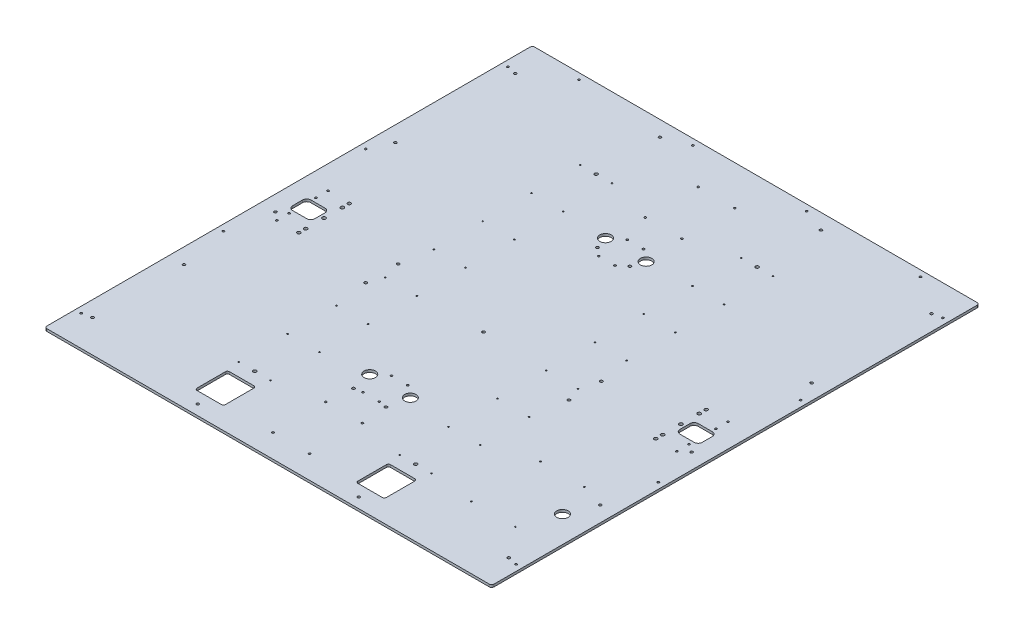
SolidWorks part; units mm, degrees
material "A3钢"
ref_plane "前视基准面" through (0, 0, 0) normal (0, 0, 1) x (1, 0, 0)
ref_plane "上视基准面" through (0, 0, 0) normal (0, 1, 0) x (1, 0, 0)
ref_plane "右视基准面" through (0, 0, 0) normal (1, 0, 0) x (0, 0, -1)
sketch "草图1" plane through (0, 0, 0) normal (0, 1, 0) x (1, 0, 0)
  line L1 (-550, 600) -> (550, 600)
  line L2 (-550, 600) -> (-550, -600)
  line L3 (-550, -600) -> (550, -600)
  line L4 (550, 600) -> (550, -600)
  line L5 (-550, 600) -> (550, -600) construction
  line L6 (-550, -600) -> (550, 600) construction
  point P0 (0, 0)
  dimension "D1" = 1100
  dimension "D2" = 1200
extrude "凸台-拉伸1" add sketch "草图1" along normal blind 6
fillet "圆角1" radius 6 4 edges at (-550, 3, -600) (550, 3, -600) (550, 3, 600) (-550, 3, 600)
hole_wizard "M6 螺纹孔1" positions "草图48" profile "草图50" tap size "M6" standard "GB" end condition through all
sketch "草图48" plane through (0, 0, 0) normal (0, -1, 0) x (-1, 0, 0)
  circle A0 centre (492, 39.5) radius 3.25 construction
  circle A1 centre (492, 9.5) radius 3.25 construction
  circle A2 centre (492, -56.5) radius 3.5 construction
  circle A3 centre (492, -86.5) radius 3.5 construction
  point P0 (492, -86.5)
  point P2 (492, -56.5)
  point P4 (492, 9.5)
  point P6 (492, 39.5)
sketch "草图50" plane through (-492, 0, 86.5) normal (1, 0, 0) x (0, 0, -1)
  line L0 (0, 0) -> (0, 6)
  line L1 (0, 6) -> (2.5, 6)
  line L2 (2.5, 6) -> (2.5, 0)
  line L5 (2.5, 0) -> (0, 0)
  line L11 (0, -6.35) -> (0, 107.95) construction
  dimension "通孔螺纹孔钻头直径" = 5
  dimension "通孔螺纹孔钻头深度" = 6
cosmetic thread "孔螺蚊线36" parameters "D2"=6
cosmetic thread "孔螺蚊线37" parameters "D2"=6
cosmetic thread "孔螺蚊线38" parameters "D2"=6
cosmetic thread "孔螺蚊线39" parameters "D2"=6
hole_wizard "Ø8.0 (8) 直径孔1" positions "草图51" profile "草图53" hole size "Ø8.0" standard "GB" end condition through all
sketch "草图51" plane through (0, 0, 0) normal (0, -1, 0) x (-1, 0, 0)
  point P0 (439, -85.5)
  point P3 (439, 38.5)
sketch "草图53" plane through (-439, 0, 85.5) normal (1, 0, 0) x (0, 0, -1)
  line L0 (0, 0) -> (0, 6)
  line L1 (0, 6) -> (4, 6)
  line L2 (4, 6) -> (4, 0)
  line L5 (4, 0) -> (0, 0)
  line L11 (0, -6.35) -> (0, 107.95) construction
  dimension "通孔孔直径" = 8
  dimension "通孔孔深度" = 6
hole_wizard "Ø8.5 (8.5) 直径孔1" positions "草图54" profile "草图55" hole size "Ø8.5" standard "GB" end condition through all
sketch "草图54" plane through (0, 0, 0) normal (0, -1, 0) x (-1, 0, 0)
  circle A0 centre (439, -68.5) radius 3.4 construction
  circle A1 centre (439, 21.5) radius 3.4 construction
  circle A2 centre (439, -23.5) radius 3.4 construction
  point P0 (439, 21.5)
  point P2 (439, -23.5)
  point P4 (439, -68.5)
sketch "草图55" plane through (-439, 0, -21.5) normal (1, 0, 0) x (0, 0, -1)
  line L0 (0, 0) -> (0, 6)
  line L1 (0, 6) -> (4.25, 6)
  line L2 (4.25, 6) -> (4.25, 0)
  line L5 (4.25, 0) -> (0, 0)
  line L11 (0, -6.35) -> (0, 107.95) construction
  dimension "通孔孔直径" = 8.5
  dimension "通孔孔深度" = 6
sketch "草图56" plane through (0, 6, 0) normal (0, 1, 0) x (1, 0, 0)
  line L0 (-439, -23.5) -> (-595.6745, -23.5) construction
  line L2 (-494, -1) -> (-459, -1)
  line L3 (-504, -11) -> (-504, -36)
  line L4 (-494, -46) -> (-459, -46)
  line L5 (-449, -11) -> (-449, -36)
  line L6 (-504, -1) -> (-449, -46) construction
  line L7 (-504, -46) -> (-449, -1) construction
  circle A0 centre (-439, -23.5) radius 4.25 construction
  arc A1 (-459, -1) -> (-449, -11) centre (-459, -11) cw
  arc A2 (-449, -36) -> (-459, -46) centre (-459, -36) cw
  arc A3 (-494, -46) -> (-504, -36) centre (-494, -36) cw
  arc A4 (-504, -11) -> (-494, -1) centre (-494, -11) cw
  point P3 (-476.5, -23.5)
  dimension "D4" = 10
  dimension "D1" = 10
  dimension "D2" = 55
  dimension "D3" = 45
extrude "切除-拉伸1" cut sketch "草图56" against normal blind 10
hole_wizard "Ø8.0 (8) 直径孔2" positions "草图63" profile "草图64" hole size "Ø8.0" standard "GB" end condition through all
sketch "草图63" plane through (0, 6, 0) normal (0, 1, 0) x (1, 0, 0)
  circle A0 centre (-198, 405) radius 4 construction
  circle A1 centre (-198, -435) radius 4 construction
  point P2 (-198, 405)
  point P7 (-198, -435)
sketch "草图64" plane through (-198, 6, -405) normal (1, 0, 0) x (0, 0, 1)
  line L0 (0, 0) -> (0, 6)
  line L1 (0, 6) -> (4, 6)
  line L2 (4, 6) -> (4, 0)
  line L5 (4, 0) -> (0, 0)
  line L11 (0, -6.35) -> (0, 107.95) construction
  dimension "通孔孔直径" = 8
  dimension "通孔孔深度" = 6
hole_wizard "M4 螺纹孔1" positions "草图65" profile "草图67" tap size "M4" standard "GB" end condition through all
sketch "草图65" plane through (0, 6, 0) normal (0, 1, 0) x (1, 0, 0)
  circle A0 centre (-237, -435) radius 2.25 construction
  circle A1 centre (-159, -435) radius 2.25 construction
  point P0 (-159, -435)
  point P2 (-237, -435)
sketch "草图67" plane through (-159, 6, 435) normal (1, 0, 0) x (0, 0, 1)
  line L0 (0, 0) -> (0, 6)
  line L1 (0, 6) -> (1.65, 6)
  line L2 (1.65, 6) -> (1.65, 0)
  line L5 (1.65, 0) -> (0, 0)
  line L11 (0, -6.35) -> (0, 107.95) construction
  dimension "通孔螺纹孔钻头直径" = 3.3
  dimension "通孔螺纹孔钻头深度" = 6
cosmetic thread "孔螺蚊线44" parameters "D2"=4
cosmetic thread "孔螺蚊线45" parameters "D2"=4
pattern_linear "阵列(线性)1" count 8 spacing 120 along (0, 0, -1) of "M4 螺纹孔1"
sketch "草图59" plane through (0, 6, 0) normal (0, 1, 0) x (1, 0, 0)
  line L0 (0, 0) -> (0, -646.723) construction
  line L1 (-544, -600) -> (544, -600) construction
  line L2 (-228, -467) -> (-168, -467)
  line L3 (-233, -472) -> (-233, -542)
  line L4 (-228, -547) -> (-168, -547)
  line L5 (-163, -472) -> (-163, -542)
  line L6 (-233, -467) -> (-163, -547) construction
  line L7 (-233, -547) -> (-163, -467) construction
  arc A0 (-168, -467) -> (-163, -472) centre (-168, -472) cw
  arc A1 (-163, -542) -> (-168, -547) centre (-168, -542) cw
  arc A2 (-228, -547) -> (-233, -542) centre (-228, -542) cw
  arc A3 (-233, -472) -> (-228, -467) centre (-228, -472) cw
  point P3 (-198, -507)
  dimension "D5" = 5
  dimension "D1" = 198
  dimension "D2" = 53
  dimension "D3" = 70
  dimension "D4" = 80
extrude "切除-拉伸2" cut sketch "草图59" against normal blind 10
mirror "镜向1" about plane through (0, 0, 0) normal (1, 0, 0) of "切除-拉伸2", "阵列(线性)1", "Ø8.0 (8) 直径孔2", "切除-拉伸1", "Ø8.5 (8.5) 直径孔1", "Ø8.0 (8) 直径孔1", "M6 螺纹孔1", "M4 螺纹孔1"
hole_wizard "M8 螺纹孔4" positions "草图57" profile "草图58" tap size "M8" standard "GB" end condition through all
sketch "草图57" plane through (0, 0, 0) normal (0, -1, 0) x (-1, 0, 0)
  point P10 (250, -30)
  point P12 (250, -110)
  point P14 (-250, -110)
  point P16 (-250, -30)
sketch "草图58" plane through (-250, 0, 30) normal (1, 0, 0) x (0, 0, -1)
  line L0 (0, 0) -> (0, 6)
  line L1 (0, 6) -> (3.4, 6)
  line L2 (3.4, 6) -> (3.4, 0)
  line L5 (3.4, 0) -> (0, 0)
  line L11 (0, -6.35) -> (0, 107.95) construction
  dimension "通孔螺纹孔钻头直径" = 6.8
  dimension "通孔螺纹孔钻头深度" = 6
cosmetic thread "孔螺蚊线40" parameters "D2"=8
cosmetic thread "孔螺蚊线41" parameters "D2"=8
cosmetic thread "孔螺蚊线42" parameters "D2"=8
cosmetic thread "孔螺蚊线43" parameters "D2"=8
hole_wizard "Ø6.5 (6.5) 直径孔1" positions "草图68" profile "草图70" hole size "Ø6.5" standard "GB" end condition through all
sketch "草图68" plane through (0, 6, 0) normal (0, 1, 0) x (1, 0, 0)
  line L0 (-550, 594) -> (-550, -594) construction
  line L1 (-544, -600) -> (544, -600) construction
  line L2 (544, 600) -> (-544, 600) construction
  line L3 (-250, -30) -> (-250, -110) construction
  line L5 (-250, -70) -> (-512, -70) construction
  line L6 (-512, -520) -> (-512, -70) construction
  line L7 (-512, 520) -> (-512, -70) construction
  point P0 (-512, -520)
  point P7 (-512, 520)
  point P20 (-512, -70)
  point P35 (-512, -295)
  point P42 (-512, 225)
  dimension "D1" = 38
  dimension "D2" = 80
  dimension "D3" = 80
sketch "草图70" plane through (-512, 6, 520) normal (1, 0, 0) x (0, 0, 1)
  line L0 (0, 0) -> (0, 6)
  line L1 (0, 6) -> (3.25, 6)
  line L2 (3.25, 6) -> (3.25, 0)
  line L5 (3.25, 0) -> (0, 0)
  line L11 (0, -6.35) -> (0, 107.95) construction
  dimension "通孔孔直径" = 6.5
  dimension "通孔孔深度" = 6
mirror "镜向2" about plane through (0, 0, 0) normal (1, 0, 0) of "Ø6.5 (6.5) 直径孔1"
hole_wizard "Ø6.5 (6.5) 直径孔2" positions "草图71" profile "草图72" hole size "Ø6.5" standard "GB" end condition through all
sketch "草图71" plane through (0, 6, 0) normal (0, 1, 0) x (1, 0, 0)
  line L0 (-250, -30) -> (-250, -110) construction
  line L2 (-250, -70) -> (43.0975, -70) construction
  line L4 (0, 0) -> (0, -761.1687) construction
  line L5 (544, 600) -> (-544, 600) construction
  line L6 (-544, -600) -> (544, -600) construction
  point P16 (0, -70)
  point P18 (-198, 562)
  point P24 (198, -575)
  point P31 (198, 562)
  point P35 (-198, -575)
  dimension "D1" = 38
  dimension "D2" = 25
  dimension "D3" = 396
  dimension "D4" = 396
sketch "草图72" plane through (-198, 6, 575) normal (1, 0, 0) x (0, 0, 1)
  line L0 (0, 0) -> (0, 6)
  line L1 (0, 6) -> (3.25, 6)
  line L2 (3.25, 6) -> (3.25, 0)
  line L5 (3.25, 0) -> (0, 0)
  line L11 (0, -6.35) -> (0, 107.95) construction
  dimension "通孔孔直径" = 6.5
  dimension "通孔孔深度" = 6
hole_wizard "M8 螺纹孔5" positions "草图75" profile "草图76" tap size "M8" standard "GB" end condition through all
sketch "草图75" plane through (0, 0, 0) normal (0, -1, 0) x (-1, 0, 0)
  point P3 (-40, 250)
  point P5 (40, 250)
  point P7 (-40, -350)
  point P9 (40, -350)
sketch "草图76" plane through (40, 0, -250) normal (1, 0, 0) x (0, 0, -1)
  line L0 (0, 0) -> (0, 6)
  line L1 (0, 6) -> (3.4, 6)
  line L2 (3.4, 6) -> (3.4, 0)
  line L5 (3.4, 0) -> (0, 0)
  line L11 (0, -6.35) -> (0, 107.95) construction
  dimension "通孔螺纹孔钻头直径" = 6.8
  dimension "通孔螺纹孔钻头深度" = 6
cosmetic thread "孔螺蚊线46" parameters "D2"=8
cosmetic thread "孔螺蚊线47" parameters "D2"=8
cosmetic thread "孔螺蚊线48" parameters "D2"=8
cosmetic thread "孔螺蚊线49" parameters "D2"=8
hole_wizard "Ø6.5 (6.5) 直径孔3" positions "草图77" profile "草图78" tap size "M6" standard "GB" end condition through all
sketch "草图77" plane through (0, 6, 0) normal (0, 1, 0) x (1, 0, 0)
  line L1 (0, 0) -> (0, -986.3558) construction
  arc A0 (-534.6942, -528.1854) -> (-534.6942, -521.8146) centre (-535, -525) ccw construction
  arc A1 (-534.6942, -178.1854) -> (-534.6942, -171.8146) centre (-535, -175) ccw construction
  arc A2 (-534.6942, 171.8146) -> (-534.6942, 178.1854) centre (-535, 175) ccw construction
  arc A3 (-534.6942, 521.8146) -> (-534.6942, 528.1854) centre (-535, 525) ccw construction
  arc A4 (-136.8146, 585.3058) -> (-143.1854, 585.3058) centre (-140, 585) ccw construction
  arc A5 (143.1854, 585.3058) -> (136.8146, 585.3058) centre (140, 585) ccw construction
  arc A6 (423.1854, 585.3058) -> (416.8146, 585.3058) centre (420, 585) ccw construction
  arc A7 (-423.1854, 584.6942) -> (-416.8146, 584.6942) centre (-420, 585) ccw construction
  point P0 (-535, 525)
  point P2 (-535, 175)
  point P4 (-535, -175)
  point P6 (-535, -525)
  point P32 (535, -525)
  point P33 (535, -175)
  point P34 (535, 175)
  point P35 (535, 525)
  point P36 (-140, 585)
  point P38 (140, 585)
  point P49 (-420, 585)
  point P57 (420, 585)
sketch "草图78" plane through (-535, 6, -525) normal (1, 0, 0) x (0, 0, 1)
  line L0 (0, 0) -> (0, 6)
  line L1 (0, 6) -> (2.5, 6)
  line L2 (2.5, 6) -> (2.5, 0)
  line L5 (2.5, 0) -> (0, 0)
  line L11 (0, -6.35) -> (0, 107.95) construction
  dimension "通孔螺纹孔钻头直径" = 5
  dimension "通孔螺纹孔钻头深度" = 6
cosmetic thread "孔螺蚊线54" parameters "D2"=6
cosmetic thread "孔螺蚊线55" parameters "D2"=6
cosmetic thread "孔螺蚊线56" parameters "D2"=6
cosmetic thread "孔螺蚊线57" parameters "D2"=6
cosmetic thread "孔螺蚊线58" parameters "D2"=6
cosmetic thread "孔螺蚊线59" parameters "D2"=6
cosmetic thread "孔螺蚊线60" parameters "D2"=6
cosmetic thread "孔螺蚊线61" parameters "D2"=6
cosmetic thread "孔螺蚊线62" parameters "D2"=6
cosmetic thread "孔螺蚊线63" parameters "D2"=6
cosmetic thread "孔螺蚊线64" parameters "D2"=6
cosmetic thread "孔螺蚊线65" parameters "D2"=6
hole_wizard "M4 螺纹孔2" positions "草图79" profile "草图81" tap size "M4" standard "GB" end condition through all
sketch "草图79" plane through (0, 6, 0) normal (0, 1, 0) x (1, 0, 0)
  line L0 (346, -455.9298) -> (346, -435.9298) construction
  line L2 (454, -455.9298) -> (454, -435.9298) construction
  line L4 (454, -263.7798) -> (454, -288.0798) construction
  line L6 (346, -265.9298) -> (346, -285.9298) construction
  arc A0 (456.15, -265.9298) -> (451.85, -265.9298) centre (454, -265.9298) ccw construction
  arc A1 (451.85, -285.9298) -> (456.15, -285.9298) centre (454, -285.9298) ccw construction
  point P0 (454, -275.9298)
  point P2 (454, -445.9298)
  point P4 (346, -445.9298)
  point P6 (346, -275.9298)
sketch "草图81" plane through (454, 6, 275.9298) normal (1, 0, 0) x (0, 0, 1)
  line L0 (0, 0) -> (0, 6)
  line L1 (0, 6) -> (1.65, 6)
  line L2 (1.65, 6) -> (1.65, 0)
  line L5 (1.65, 0) -> (0, 0)
  line L11 (0, -6.35) -> (0, 107.95) construction
  dimension "通孔螺纹孔钻头直径" = 3.3
  dimension "通孔螺纹孔钻头深度" = 6
cosmetic thread "孔螺蚊线50" parameters "D1"=6, "D2"=4
cosmetic thread "孔螺蚊线51" parameters "D1"=6, "D2"=4
cosmetic thread "孔螺蚊线52" parameters "D1"=6, "D2"=4
cosmetic thread "孔螺蚊线53" parameters "D1"=6, "D2"=4
sketch "草图82" plane through (0, 6, 0) normal (0, 1, 0) x (1, 0, 0)
  line L0 (346, -445.9298) -> (454, -275.9298) construction
  line L1 (400, -360.9298) -> (485, -360.9298) construction
  circle A3 centre (485, -360.9298) radius 14
  dimension "D1" = 28
  dimension "D2" = 85
extrude "切除-拉伸3" cut sketch "草图82" against normal blind 10
hole_wizard "M6 螺纹孔2" positions "草图83" profile "草图84" tap size "M6" standard "GB" end condition through all
sketch "草图83" plane through (0, 6, 0) normal (0, 1, 0) x (1, 0, 0)
  line L0 (-45, -399.75) -> (-45, -426.25) construction
  line L2 (45, -399.75) -> (45, -426.25) construction
  line L4 (-45, -556.25) -> (-45, -529.75) construction
  line L6 (45, -556.25) -> (45, -529.75) construction
  line L8 (20, -333.25) -> (20, -359.75) construction
  line L10 (-20, -333.25) -> (-20, -359.75) construction
  line L12 (-20, -263.25) -> (-20, -289.75) construction
  line L14 (20, -263.25) -> (20, -289.75) construction
  line L16 (-45, 386.25) -> (-45, 359.75) construction
  line L18 (45, 386.25) -> (45, 359.75) construction
  line L20 (-45, 516.25) -> (-45, 489.75) construction
  line L22 (45, 516.25) -> (45, 489.75) construction
  line L23 (-20, 223.5) -> (-20, 243.5) construction
  line L25 (20, 243.5) -> (20, 223.5) construction
  line L27 (-20, 313.5) -> (-20, 293.5) construction
  line L29 (20, 313.5) -> (20, 293.5) construction
  arc A0 (-41.75, -403) -> (-48.25, -403) centre (-45, -403) ccw construction
  arc A1 (-48.25, -423) -> (-41.75, -423) centre (-45, -423) ccw construction
  arc A2 (48.25, -403) -> (41.75, -403) centre (45, -403) ccw construction
  arc A3 (41.75, -423) -> (48.25, -423) centre (45, -423) ccw construction
  arc A4 (-48.25, -553) -> (-41.75, -553) centre (-45, -553) ccw construction
  arc A5 (-41.75, -533) -> (-48.25, -533) centre (-45, -533) ccw construction
  arc A6 (41.75, -553) -> (48.25, -553) centre (45, -553) ccw construction
  arc A7 (48.25, -533) -> (41.75, -533) centre (45, -533) ccw construction
  arc A8 (23.25, -336.5) -> (16.75, -336.5) centre (20, -336.5) ccw construction
  arc A9 (16.75, -356.5) -> (23.25, -356.5) centre (20, -356.5) ccw construction
  arc A10 (-16.75, -336.5) -> (-23.25, -336.5) centre (-20, -336.5) ccw construction
  arc A11 (-23.25, -356.5) -> (-16.75, -356.5) centre (-20, -356.5) ccw construction
  arc A12 (-16.75, -266.5) -> (-23.25, -266.5) centre (-20, -266.5) ccw construction
  arc A13 (-23.25, -286.5) -> (-16.75, -286.5) centre (-20, -286.5) ccw construction
  arc A14 (23.25, -266.5) -> (16.75, -266.5) centre (20, -266.5) ccw construction
  arc A15 (16.75, -286.5) -> (23.25, -286.5) centre (20, -286.5) ccw construction
  arc A16 (-41.75, 383) -> (-48.25, 383) centre (-45, 383) ccw construction
  arc A17 (-48.25, 363) -> (-41.75, 363) centre (-45, 363) ccw construction
  arc A18 (48.25, 383) -> (41.75, 383) centre (45, 383) ccw construction
  arc A19 (41.75, 363) -> (48.25, 363) centre (45, 363) ccw construction
  arc A20 (-41.75, 513) -> (-48.25, 513) centre (-45, 513) ccw construction
  arc A21 (-48.25, 493) -> (-41.75, 493) centre (-45, 493) ccw construction
  arc A22 (48.25, 513) -> (41.75, 513) centre (45, 513) ccw construction
  arc A23 (41.75, 493) -> (48.25, 493) centre (45, 493) ccw construction
  point P116 (-45, -413)
  point P118 (-45, -543)
  point P120 (45, -413)
  point P122 (45, -543)
  point P124 (20, -276.5)
  point P126 (20, -346.5)
  point P128 (-20, -276.5)
  point P130 (-20, -346.5)
  point P132 (20, 303.5)
  point P134 (20, 233.5)
  point P136 (-20, 303.5)
  point P138 (-20, 233.5)
  point P140 (-45, 503)
  point P142 (-45, 373)
  point P144 (45, 503)
  point P146 (45, 373)
sketch "草图84" plane through (45, 6, -373) normal (1, 0, 0) x (0, 0, 1)
  line L0 (0, 0) -> (0, 6)
  line L1 (0, 6) -> (2.5, 6)
  line L2 (2.5, 6) -> (2.5, 0)
  line L5 (2.5, 0) -> (0, 0)
  line L11 (0, -6.35) -> (0, 107.95) construction
  dimension "通孔螺纹孔钻头直径" = 5
  dimension "通孔螺纹孔钻头深度" = 6
cosmetic thread "孔螺蚊线66" parameters "D2"=6
cosmetic thread "孔螺蚊线67" parameters "D2"=6
cosmetic thread "孔螺蚊线68" parameters "D2"=6
cosmetic thread "孔螺蚊线69" parameters "D2"=6
cosmetic thread "孔螺蚊线70" parameters "D2"=6
cosmetic thread "孔螺蚊线71" parameters "D2"=6
cosmetic thread "孔螺蚊线72" parameters "D2"=6
cosmetic thread "孔螺蚊线73" parameters "D2"=6
cosmetic thread "孔螺蚊线74" parameters "D2"=6
cosmetic thread "孔螺蚊线75" parameters "D2"=6
cosmetic thread "孔螺蚊线76" parameters "D2"=6
cosmetic thread "孔螺蚊线77" parameters "D2"=6
cosmetic thread "孔螺蚊线78" parameters "D2"=6
cosmetic thread "孔螺蚊线79" parameters "D2"=6
cosmetic thread "孔螺蚊线80" parameters "D2"=6
cosmetic thread "孔螺蚊线81" parameters "D2"=6
sketch "草图86" plane through (0, 6, 0) normal (0, 1, 0) x (1, 0, 0)
  line L0 (0, 0) -> (0, 728.4781) construction
  circle A0 centre (50, 280) radius 14
  circle A1 centre (-50, 280) radius 14
  circle A2 centre (50, -300) radius 14
  circle A3 centre (-50, -300) radius 14
  dimension "D1" = 28
  dimension "D2" = 28
  dimension "D4" = 300
  dimension "D5" = 28
  dimension "D3" = 100
  dimension "D6" = 280
  dimension "D7" = 100
extrude "切除-拉伸4" cut sketch "草图86" against normal blind 10
